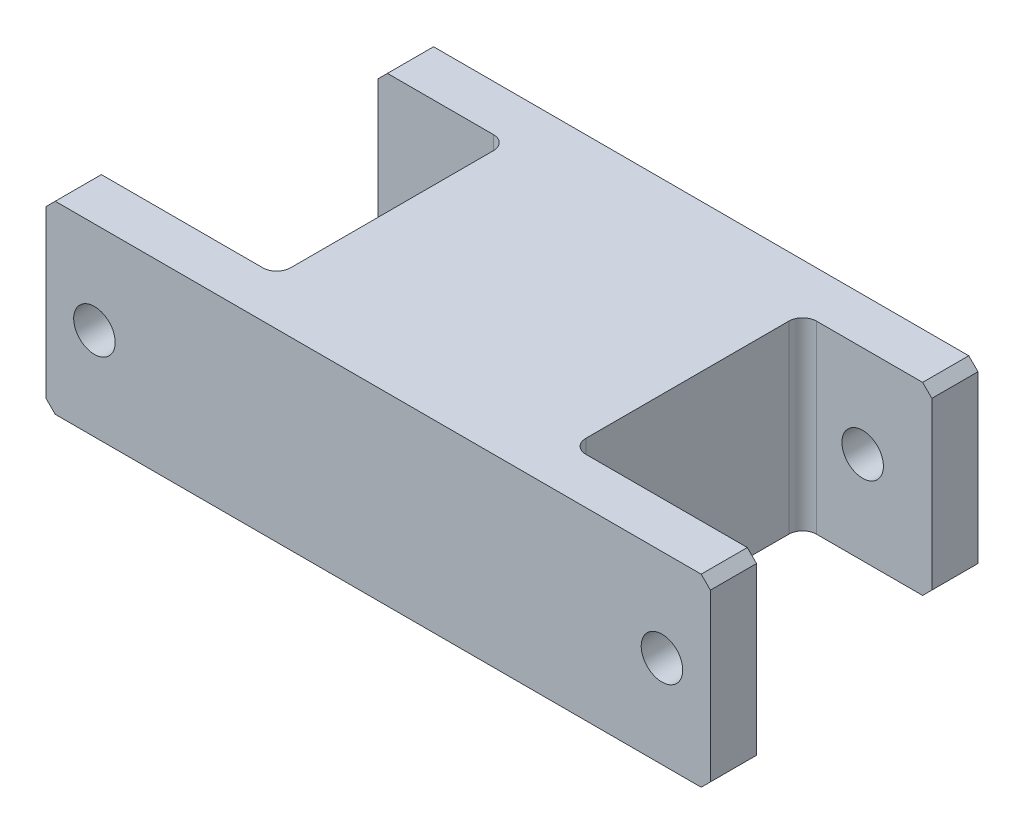
SolidWorks part; units mm, degrees
material "AISI 1045 钢，冷拔"
ref_plane "前视基准面" through (0, 0, 0) normal (0, 0, 1) x (1, 0, 0)
ref_plane "上视基准面" through (0, 0, 0) normal (0, 1, 0) x (1, 0, 0)
ref_plane "右视基准面" through (0, 0, 0) normal (1, 0, 0) x (0, 0, -1)
sketch "草图1" plane through (0, 0, 0) normal (0, 0, 1) x (1, 0, 0)
  line L1 (179.2844, 44.5489) -> (59.2844, 44.5489)
  line L2 (179.2844, 44.5489) -> (179.2844, 4.5489)
  line L3 (179.2844, 4.5489) -> (59.2844, 4.5489)
  line L4 (59.2844, 44.5489) -> (59.2844, 4.5489)
  dimension "D1" = 120
  dimension "D2" = 40
extrude "凸台-拉伸1" add sketch "草图1" along normal blind 70
sketch "草图2" plane through (0, 0, 70) normal (0, 0, 1) x (1, 0, 0)
  line L0 (179.2844, 24.5489) -> (59.2844, 24.5489) construction
  line L1 (179.2844, 4.5489) -> (179.2844, 44.5489) construction
  line L2 (59.2844, 44.5489) -> (59.2844, 4.5489) construction
  circle A0 centre (119.2844, 24.5489) radius 45 construction
  circle A1 centre (74.2844, 24.5489) radius 3
  circle A2 centre (164.2844, 24.5489) radius 3
  dimension "D1" = 90
  dimension "D2" = 6
extrude "切除-拉伸1" cut sketch "草图2" against normal through all
sketch "草图3" plane through (0, 44.5489, 0) normal (0, 1, 0) x (1, 0, 0)
  line L0 (119.2844, -70) -> (119.2844, 0) construction
  line L1 (179.2844, -70) -> (59.2844, -70) construction
  line L2 (179.2844, 0) -> (59.2844, 0) construction
  line L3 (179.2844, -35) -> (53.3553, -35) construction
  line L4 (151.2844, -60) -> (198.6079, -60)
  line L5 (151.2844, -60) -> (151.2844, -10)
  line L6 (151.2844, -10) -> (198.6079, -10)
  line L7 (198.6079, -60) -> (198.6079, -10)
  line L8 (179.2844, -70) -> (179.2844, 0) construction
  line L9 (87.2844, -60) -> (87.2844, -10)
  line L10 (39.961, -60) -> (39.961, -10)
  line L11 (87.2844, -10) -> (39.961, -10)
  line L12 (87.2844, -60) -> (39.961, -60)
  dimension "D1" = 10
  dimension "D2" = 32
extrude "切除-拉伸2" cut sketch "草图3" against normal through all
fillet "圆角1" radius 3 4 edges at (87.2844, 24.5489, 10) (151.2844, 24.5489, 10) (87.2844, 24.5489, 60) (151.2844, 24.5489, 60)
sketch "草图4" plane through (0, 0, 60) normal (0, 0, -1) x (-1, 0, 0)
  line L0 (-59.2844, 44.5489) -> (-84.2844, 44.5489) construction
  line L1 (-179.2844, 4.5489) -> (-191.2844, 4.5489)
  line L2 (-179.2844, 4.5489) -> (-179.2844, 44.5489)
  line L3 (-179.2844, 44.5489) -> (-191.2844, 44.5489)
  line L4 (-191.2844, 4.5489) -> (-191.2844, 44.5489)
  dimension "D1" = 12
extrude "凸台-拉伸2" add sketch "草图4" against normal up to vertex (10 mm away) up to point (179.2844, 4.5489, 70)
ref_plane "基准面1" through (119.2844, 0, 0) normal (1, 0, 0) x (0, 0, -1)
sketch "草图5" plane through (0, 0, 70) normal (0, 0, 1) x (1, 0, 0)
  line L0 (59.2844, 4.5489) -> (191.2844, 4.5489) construction
  line L1 (59.2844, 44.5489) -> (47.2844, 44.5489)
  line L2 (59.2844, 44.5489) -> (59.2844, 4.5489)
  line L3 (59.2844, 4.5489) -> (47.2844, 4.5489)
  line L4 (47.2844, 44.5489) -> (47.2844, 4.5489)
  dimension "D1" = 12
extrude "凸台-拉伸3" add sketch "草图5" against normal up to surface (10 mm away) up to face at (77.2844, 24.5489, 60)
sketch "草图6" plane through (0, 0, 70) normal (0, 0, 1) x (1, 0, 0)
  circle A0 centre (74.2844, 24.5489) radius 3 construction
  circle A1 centre (74.2844, 24.5489) radius 3
  circle A2 centre (164.2844, 24.5489) radius 3 construction
  circle A3 centre (164.2844, 24.5489) radius 3
extrude "凸台-拉伸4" add sketch "草图6" against normal up to surface (10 mm away) up to face at (77.2844, 24.5489, 60)
sketch "草图7" plane through (0, 0, 70) normal (0, 0, 1) x (1, 0, 0)
  line L0 (74.2844, 24.5489) -> (57.7844, 24.5489) construction
  circle A0 centre (57.7844, 24.5489) radius 4.5
  dimension "D1" = 9
  dimension "D2" = 16.5
extrude "切除-拉伸3" cut sketch "草图7" against normal up to surface (10 mm away) up to face at (65.7844, 24.5489, 60)
mirror "镜向2" about plane through (119.2844, 0, 0) normal (1, 0, 0) of "切除-拉伸3"
sketch "草图8" [suppressed] plane through (0, 44.5489, 0) normal (0, 1, 0) x (1, 0, 0)
  line L0 (109.2844, -42) -> (109.2844, -12) construction
sketch "草图10" plane through (0, 44.5489, 0) normal (0, 1, 0) x (1, 0, 0)
  line L0 (109.2844, -62) -> (109.2844, -32) construction
  line L1 (87.2844, -57) -> (87.2844, -13) construction
  line L2 (191.2844, -70) -> (47.2844, -70) construction
  dimension "D1" = 22
  dimension "D2" = 8
  dimension "D3" = 30
hole_wizard "M10 螺纹孔1" positions "3D草图1" profile "草图9" tap size "M10" standard "GB"
sketch3d "3D草图1" [suppressed]
  point P0 (109.2844, 44.5489, 42)
  point P3 (109.2844, 44.5489, 12)
sketch "草图9" plane through (109.2844, 44.5489, 42) normal (1, 0, 0) x (0, 0, 1)
  line L0 (0, 0) -> (0, 26.5537)
  line L1 (0, 26.5537) -> (4.25, 24)
  line L2 (4.25, 24) -> (4.25, 0)
  line L5 (4.25, 0) -> (0, 0)
  line L10 (0, 26.5537) -> (-4.25, 24) construction
  line L11 (0, -6.35) -> (0, 107.95) construction
  dimension "螺纹孔钻头直径" = 8.5
  dimension "螺纹孔钻头深度" = 24
  dimension "导头角度" = 118
hole_wizard "M8 螺纹孔1" positions "3D草图2" profile "草图11" tap size "M8" standard "GB"
sketch3d "3D草图2"
  point P0 (109.2844, 44.5489, 52)
  point P3 (109.2844, 44.5489, 22)
sketch "草图11" plane through (109.2844, 44.5489, 52) normal (1, 0, 0) x (0, 0, 1)
  line L0 (0, 0) -> (0, 21.7929)
  line L1 (0, 21.7929) -> (3.4, 19.75)
  line L2 (3.4, 19.75) -> (3.4, 0)
  line L5 (3.4, 0) -> (0, 0)
  line L10 (0, 21.7929) -> (-3.4, 19.75) construction
  line L11 (0, -6.35) -> (0, 107.95) construction
  dimension "螺纹孔钻头直径" = 6.8
  dimension "螺纹孔钻头深度" = 19.75
  dimension "导头角度" = 118
cosmetic thread "孔螺蚊线1" [suppressed] parameters "D1"=16, "D2"=8
cosmetic thread "孔螺蚊线2" [suppressed] parameters "D1"=16, "D2"=8
chamfer "倒角1" distance 2 angle 45 8 edges at (59.2844, 4.5489, 5) (59.2844, 44.5489, 5) (179.2844, 44.5489, 5) (179.2844, 4.5489, 5) (191.2844, 4.5489, 65) (47.2844, 4.5489, 65) (47.2844, 44.5489, 65) (191.2844, 44.5489, 65)
hole_wizard "M8 间隙孔1" positions "3D草图3" profile "草图12" hole size "M8" standard "GB"
sketch3d "3D草图3"
  line L0 (74.2844, 24.5489, 0) -> (74.2844, 24.5489, 10) construction
  line L1 (164.2844, 24.5489, 0) -> (164.2844, 24.5489, 10) construction
  point P0 (74.2844, 24.5489, 0)
  point P4 (164.2844, 24.5489, 0)
sketch "草图12" plane through (74.2844, 24.5489, 0) normal (1, 0, 0) x (0, 1, 0)
  line L0 (0, 0) -> (0, 22.4539)
  line L1 (0, 22.4539) -> (4.5, 19.75)
  line L2 (4.5, 19.75) -> (4.5, 0)
  line L5 (4.5, 0) -> (0, 0)
  line L10 (0, 22.4539) -> (-4.5, 19.75) construction
  line L11 (0, -6.35) -> (0, 107.95) construction
  dimension "孔直径" = 9
  dimension "孔深度" = 19.75
  dimension "导头角度" = 118
